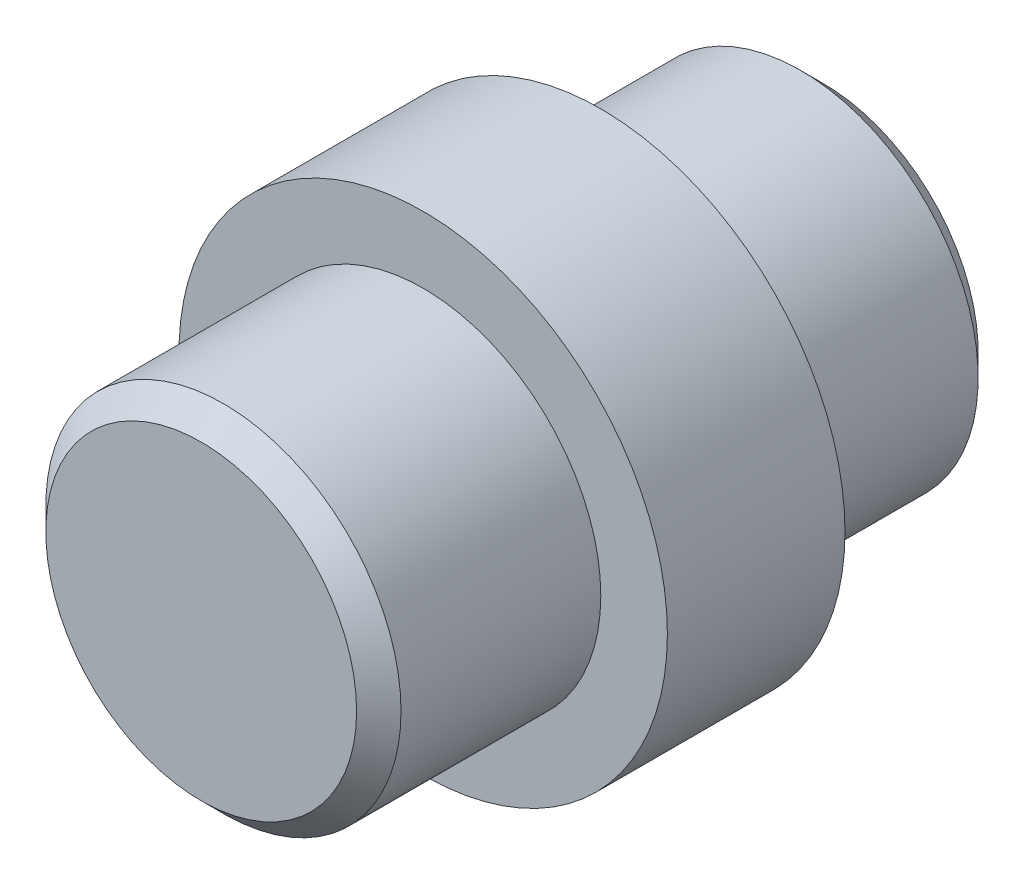
from build123d import *

# Parameters (mm, degrees)
SKETCH1_R           = 11
BOSS_EXTRUDE1_DEPTH = 8
SKETCH2_R           = 8
BOSS_EXTRUDE2_DEPTH = 10
BOSS_EXTRUDE3_START = 10
SKETCH3_R           = 8
BOSS_EXTRUDE3_DEPTH = 10
CHAMFER1_SIZE       = 1


with BuildPart() as part:
    # Sketch1 → Boss-Extrude1 (new body)
    with BuildSketch(Plane.XY):
        Circle(SKETCH1_R)
    extrude(amount=BOSS_EXTRUDE1_DEPTH)

    # Sketch2 → Boss-Extrude2 (add)
    with BuildSketch(Plane.XY.offset(8)):
        Circle(SKETCH2_R)
    extrude(amount=BOSS_EXTRUDE2_DEPTH)

    # Sketch3 → Boss-Extrude3 (add)
    with BuildSketch(Plane(origin=(0, 0, 0), x_dir=(-1, 0, 0), z_dir=(0, 0, -1)).offset(BOSS_EXTRUDE3_START)):
        with Locations(Location((0, 0, 0), (0, 0, 180))):
            Circle(SKETCH3_R)
    extrude(amount=-BOSS_EXTRUDE3_DEPTH)

    # Chamfer1
    chamfer1_edges = [part.edges().sort_by_distance(p)[0] for p in [
        (-8, 0, -10),
        (-8, 0, 18),
    ]]
    chamfer(chamfer1_edges, length=CHAMFER1_SIZE)


solid = part.part
